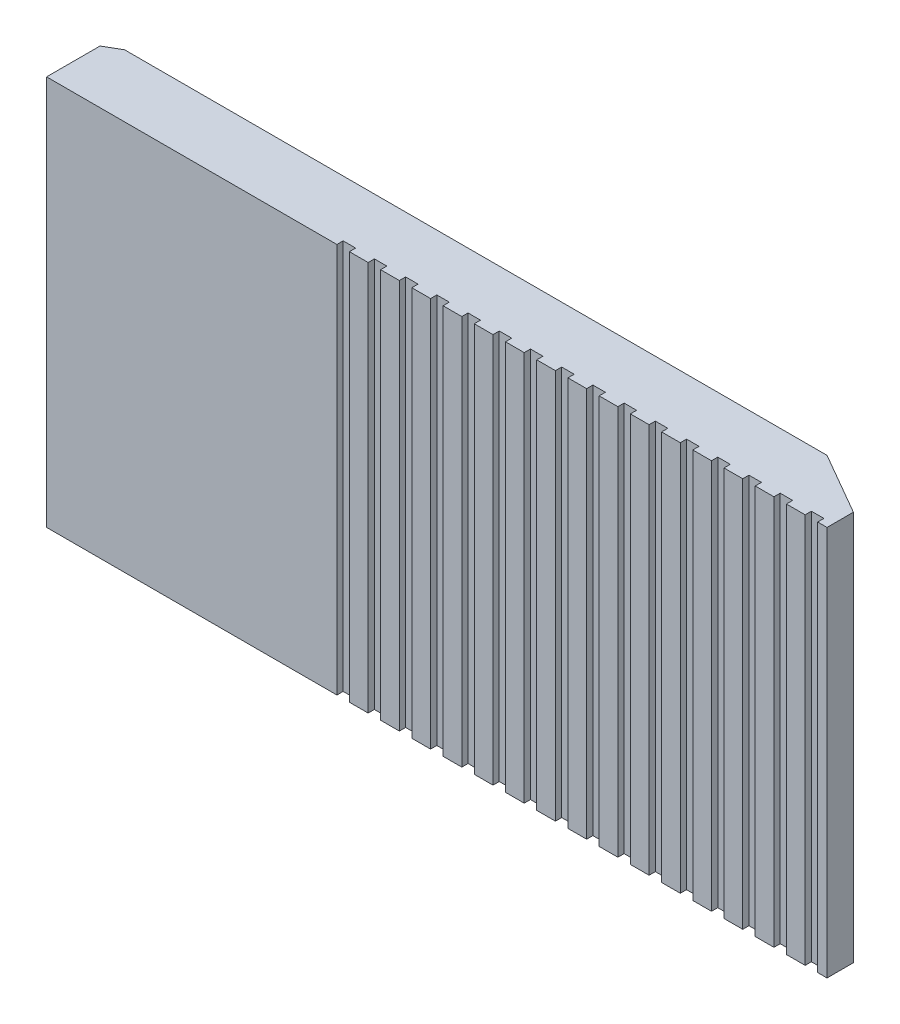
from build123d import *

# Parameters (mm, degrees)
SKETCH1_W           = 50
SKETCH1_H           = 25
BOSS_EXTRUDE1_DEPTH = 4
CHAMFER1_SIZE       = 4
CHAMFER1_SIZE2      = 2.309401077
SKETCH2_W           = 10
SKETCH2_H           = 10
BOSS_EXTRUDE2_DEPTH = 5.5
SKETCH3_W           = 0.8
SKETCH3_H           = 0.8
CUT_EXTRUDE1_DEPTH  = 36.780581326
LPATTERN1_COUNT     = 16
LPATTERN1_PITCH     = 2
CHAMFER2_SIZE       = 1
CHAMFER2_SIZE2      = 0.577350269


with BuildPart() as part:
    # Sketch1 → Boss-Extrude1 (new body)
    with BuildSketch(Plane.XY):
        Rectangle(SKETCH1_W, SKETCH1_H)
    extrude(amount=BOSS_EXTRUDE1_DEPTH)

    # Chamfer1
    chamfer1_edges = [part.edges().sort_by_distance(p)[0] for p in [
        (25, 0, 0),
    ]]
    chamfer1_side = [part.faces().sort_by_distance(p)[0] for p in [
        (0, 0, 0),
    ]]
    chamfer(chamfer1_edges, length=CHAMFER1_SIZE, length2=CHAMFER1_SIZE2, reference=chamfer1_side[0])

    # Sketch2 → Boss-Extrude2 (add)
    with BuildSketch(Plane(origin=(0, 0, 0), x_dir=(-1, 0, 0), z_dir=(0, 0, -1))):
        with Locations((-10, 0)):
            Rectangle(SKETCH2_W, SKETCH2_H)
    extrude(amount=BOSS_EXTRUDE2_DEPTH)

    # Sketch3 → Cut-Extrude1 (cut, through all)
    with BuildSketch(Plane(origin=(0, 12.5, 0), x_dir=(1, 0, 0), z_dir=(0, 1, 0))):
        with Locations((24, -4)):
            Rectangle(SKETCH3_W, SKETCH3_H)
    cut_extrude1 = extrude(amount=-CUT_EXTRUDE1_DEPTH, mode=Mode.SUBTRACT)

    # LPattern1: Cut-Extrude1 ×16
    with Locations(*[(-i * LPATTERN1_PITCH, 0, 0) for i in range(1, LPATTERN1_COUNT)]):
        add(cut_extrude1, mode=Mode.SUBTRACT)

    # Chamfer2
    chamfer2_edges = [part.edges().sort_by_distance(p)[0] for p in [
        (-25, 0, 0),
    ]]
    chamfer2_side = [part.faces().sort_by_distance(p)[0] for p in [
        (-3.142857143, 0, 0),
    ]]
    chamfer(chamfer2_edges, length=CHAMFER2_SIZE, length2=CHAMFER2_SIZE2, reference=chamfer2_side[0])


solid = part.part
